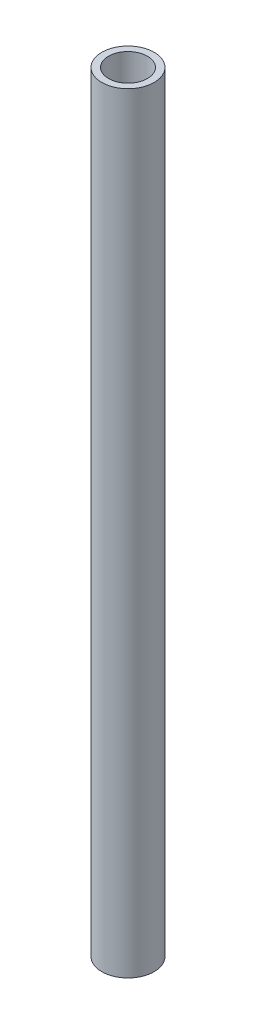
from build123d import *

# Parameters (mm, degrees)
SKETCH_1_R      = 17.5
EXTRUDE_1_DEPTH = 515
SHELL_1_T       = -4.5


with BuildPart() as part:
    # 草图1 → 凸台-拉伸1 (new body)
    with BuildSketch(Plane(origin=(0, 0, 0), x_dir=(1, 0, 0), z_dir=(0, 1, 0))):
        with Locations(Location((0, 0, 0), (0, 0, 270))):
            Circle(SKETCH_1_R)
    extrude(amount=EXTRUDE_1_DEPTH)

    # 抽壳1
    shell_1_openings = [part.faces().sort_by_distance(p)[0] for p in [
        (0, 515, 0),
        (0, 0, 0),
    ]]
    offset(amount=SHELL_1_T, openings=shell_1_openings, kind=Kind.INTERSECTION)


solid = part.part
